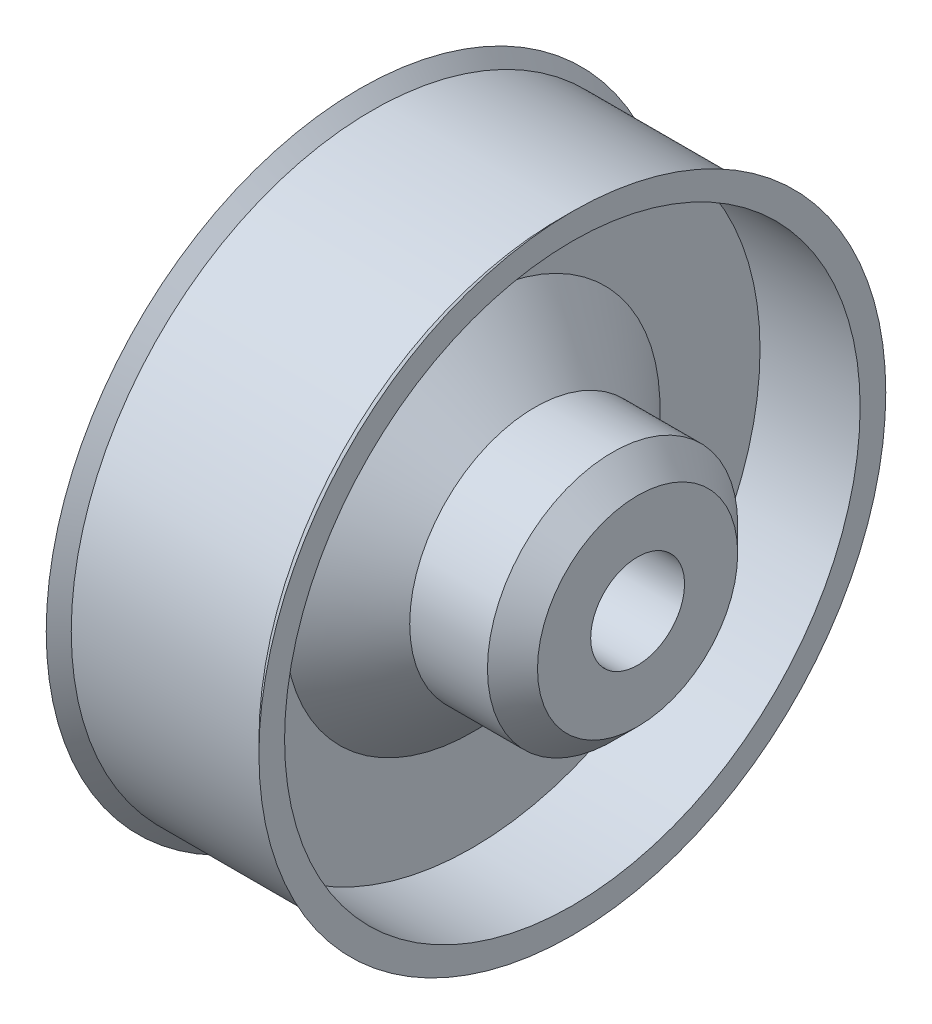
SolidWorks part; units mm, degrees
ref_plane "Front Plane" through (0, 0, 0) normal (0, 0, 1) x (1, 0, 0)
ref_plane "Top Plane" through (0, 0, 0) normal (0, 1, 0) x (1, 0, 0)
ref_plane "Right Plane" through (0, 0, 0) normal (1, 0, 0) x (0, 0, -1)
sketch "Sketch1" plane through (0, 0, 0) normal (0, 0, 1) x (1, 0, 0)
  line L0 (-4.443, 5.01) -> (-4.443, 4.6)
  line L1 (-4.443, 4.6) -> (-3.393, 4.6)
  line L2 (-3.393, 4.6) -> (-3.393, 1.248)
  line L3 (-4.443, 5.01) -> (-4.243, 4.81)
  line L4 (-4.243, 4.81) -> (-1.243, 4.81)
  line L5 (-1.243, 4.81) -> (-1.043, 5.01)
  line L6 (-1.043, 5.01) -> (-1.043, 4.6)
  line L7 (-1.043, 4.6) -> (-2.643, 4.6)
  line L8 (-2.643, 4.6) -> (-2.643, 3)
  line L9 (-2.643, 3) -> (-1.643, 2)
  line L10 (-1.643, 2) -> (-0.4, 2)
  line L11 (-0.4, 2) -> (0, 1.6)
  line L12 (0, 1.6) -> (0, 0.75)
  line L13 (0, 0.75) -> (-2.75, 0.75)
  line L14 (-2.75, 0.75) -> (-2.75, 0)
  line L15 (-3.393, 1.248) -> (-4.443, 0.8131)
  line L16 (-4.443, 0.8131) -> (-4.55, 0)
  line L17 (-2.75, 0) -> (0, 0) construction
  line L18 (-4.55, 0) -> (-2.75, 0)
  point P16 (0, 1.175)
  dimension "D2" = 1
  dimension "D3" = 1
  dimension "D4" = 0.75
  dimension "D5" = 1.8
  dimension "D6" = 4.55
  dimension "D7" = 2
  dimension "D8" = 0.75
  dimension "D9" = 1.05
  dimension "D10" = 0.4
  dimension "D11" = 0.4
  dimension "D12" = 0.2
  dimension "D13" = 7.5
  dimension "D14" = 1.157
  dimension "D15" = 4.6
  dimension "D16" = 5.01
  dimension "D17" = 3.2
revolve "Revolve1" add sketch "Sketch1" angle 360 about L17
